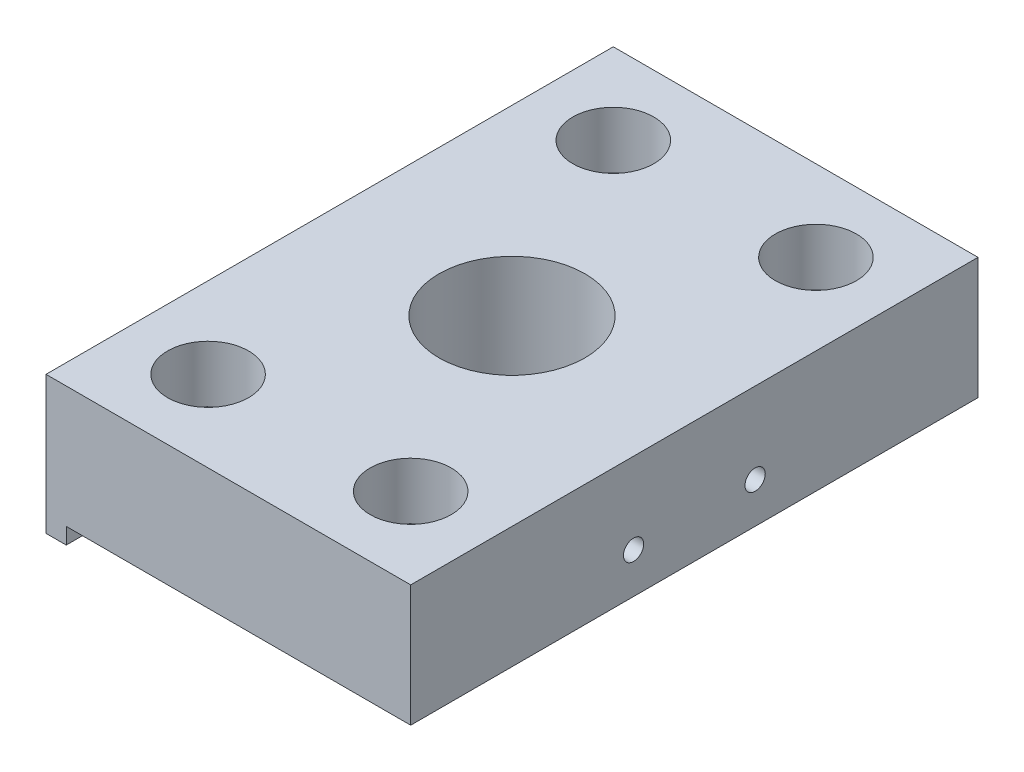
SolidWorks part; units mm, degrees
material "6061"
ref_plane "前视基准面" through (0, 0, 0) normal (0, 0, 1) x (1, 0, 0)
ref_plane "上视基准面" through (0, 0, 0) normal (0, 1, 0) x (1, 0, 0)
ref_plane "右视基准面" through (0, 0, 0) normal (1, 0, 0) x (0, 0, -1)
sketch "草图1" plane through (0, 0, 0) normal (0, 1, 0) x (1, 0, 0)
  line L1 (22.5, -35) -> (-22.5, -35)
  line L2 (22.5, -35) -> (22.5, 35)
  line L3 (22.5, 35) -> (-22.5, 35)
  line L4 (-22.5, -35) -> (-22.5, 35)
  line L5 (22.5, -35) -> (-22.5, 35) construction
  line L6 (22.5, 35) -> (-22.5, -35) construction
  point P0 (0, 0)
  dimension "D1" = 45
  dimension "D2" = 70
extrude "凸台-拉伸1" add sketch "草图1" along normal mid plane 17
sketch "草图2" plane through (0, -8.5, 0) normal (0, -1, 0) x (1, 0, 0)
  line L0 (-22.5, 35) -> (22.5, 35) construction
  line L1 (-20, 35) -> (22.5, 35)
  line L2 (-20, 35) -> (-20, -35)
  line L3 (-20, -35) -> (22.5, -35)
  line L4 (22.5, 35) -> (22.5, -35)
  dimension "D1" = 42.5
extrude "切除-拉伸1" cut sketch "草图2" against normal blind 2
hole_wizard "打孔尺寸(%根据)内六角圆柱头螺钉的类型1" positions "草图3" profile "草图4" counterbore size "M5" standard "GB" end condition through all
sketch "草图3" plane through (0, 8.5, 0) normal (0, 1, 0) x (1, 0, 0)
  line L1 (-12.5, -25) -> (12.5, -25)
  line L2 (-12.5, -25) -> (-12.5, 25)
  line L3 (-12.5, 25) -> (12.5, 25)
  line L4 (12.5, -25) -> (12.5, 25)
  line L5 (-12.5, -25) -> (12.5, 25)
  point P0 (-12.5, -25)
  point P2 (-12.5, 25)
  point P4 (12.5, 25)
  point P6 (12.5, -25)
  dimension "D1" = 50
  dimension "D2" = 25
sketch "草图4" plane through (-12.5, 8.5, 25) normal (1, 0, 0) x (0, 0, 1)
  line L0 (0, 0) -> (0, 17)
  line L1 (0, 17) -> (2.75, 17)
  line L3 (2.75, 17) -> (2.75, 7)
  line L4 (2.75, 7) -> (5, 7)
  line L5 (5, 7) -> (5, 0)
  line L7 (5, 0) -> (0, 0)
  line L11 (0, -6.35) -> (0, 107.95) construction
  dimension "通孔孔直径" = 5.5
  dimension "通孔孔深度" = 17
  dimension "柱形沉头孔直径" = 10
  dimension "柱形沉头孔深度" = 7
hole_wizard "Ø18.0 (18) 直径孔1" positions "草图5" profile "草图6" hole size "Ø18.0" standard "GB" end condition through all
sketch "草图5" plane through (0, 8.5, 0) normal (0, 1, 0) x (1, 0, 0)
  point P0 (0, 0)
sketch "草图6" plane through (0, 8.5, 0) normal (1, 0, 0) x (0, 0, 1)
  line L0 (0, 0) -> (0, 17)
  line L1 (0, 17) -> (9, 17)
  line L2 (9, 17) -> (9, 0)
  line L5 (9, 0) -> (0, 0)
  line L11 (0, -6.35) -> (0, 107.95) construction
  dimension "通孔孔直径" = 18
  dimension "通孔孔深度" = 17
hole_wizard "M3 螺纹孔1" positions "草图7" profile "草图9" tap size "M3" standard "GB"
sketch "草图7" plane through (22.5, 0, 0) normal (1, 0, 0) x (0, 0, -1)
  line L0 (-7.5, 1.5) -> (-7.5, -4.5) construction
  line L2 (7.5, 1.5) -> (7.5, -4.5) construction
  arc A0 (-5.5, -0.5) -> (-9.5, -0.5) centre (-7.5, -0.5) ccw construction
  arc A1 (-9.5, -2.5) -> (-5.5, -2.5) centre (-7.5, -2.5) ccw construction
  arc A2 (9.5, -0.5) -> (5.5, -0.5) centre (7.5, -0.5) ccw construction
  arc A3 (5.5, -2.5) -> (9.5, -2.5) centre (7.5, -2.5) ccw construction
  point P28 (7.5, -1.5)
  point P30 (-7.5, -1.5)
sketch "草图9" plane through (22.5, -1.5, -7.5) normal (0, 1, 0) x (0, 0, -1)
  line L0 (0, 0) -> (0, 9.2511)
  line L1 (0, 9.2511) -> (1.25, 8.5)
  line L2 (1.25, 8.5) -> (1.25, 0)
  line L5 (1.25, 0) -> (0, 0)
  line L10 (0, 9.2511) -> (-1.25, 8.5) construction
  line L11 (0, -6.35) -> (0, 107.95) construction
  dimension "螺纹孔钻头直径" = 2.5
  dimension "螺纹孔钻头深度" = 8.5
  dimension "导头角度" = 118
cosmetic thread "孔螺蚊线1"
cosmetic thread "孔螺蚊线2"
